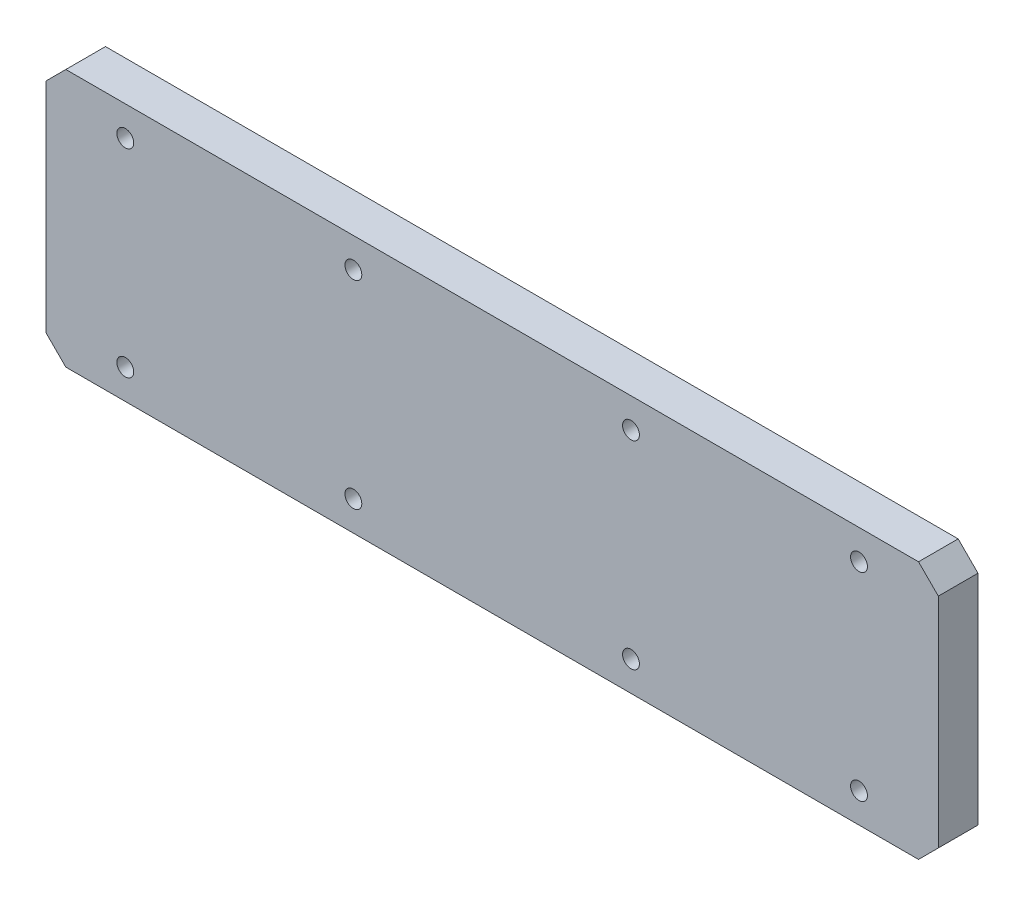
from build123d import *

# Parameters (mm, degrees)
SKETCH1_W                      = 900
SKETCH1_H                      = 260
BOSS_EXTRUDE1_DEPTH            = 40
F_17_0_17_DIAMETER_HOLE1_D     = 17
F_17_0_17_DIAMETER_HOLE1_DEPTH = 42
F_17_0_17_DIAMETER_HOLE1_TIP   = 5.107315262
CHAMFER1_SIZE                  = 20


with BuildPart() as part:
    # Sketch1 → Boss-Extrude1 (new body)
    with BuildSketch(Plane.XY):
        Rectangle(SKETCH1_W, SKETCH1_H)
    extrude(amount=BOSS_EXTRUDE1_DEPTH)

    # Ø17.0 (17) Diameter Hole1
    with Locations(Plane.XY.offset(40)):
        with Locations((-370, 100), (-140, 100), (-370, -100), (-140, -100), (140, -100), (370, -100), (140, 100), (370, 100)):
            Hole(F_17_0_17_DIAMETER_HOLE1_D / 2, depth=F_17_0_17_DIAMETER_HOLE1_DEPTH)
            with Locations((0, 0, -(F_17_0_17_DIAMETER_HOLE1_DEPTH + F_17_0_17_DIAMETER_HOLE1_TIP / 2))):  # 118° drill point
                Cone(0, F_17_0_17_DIAMETER_HOLE1_D / 2, F_17_0_17_DIAMETER_HOLE1_TIP, mode=Mode.SUBTRACT)

    # Chamfer1
    chamfer1_edges = [part.edges().sort_by_distance(p)[0] for p in [
        (-450, 130, 20),
        (450, 130, 20),
        (450, -130, 20),
        (-450, -130, 20),
    ]]
    chamfer(chamfer1_edges, length=CHAMFER1_SIZE)


solid = part.part
